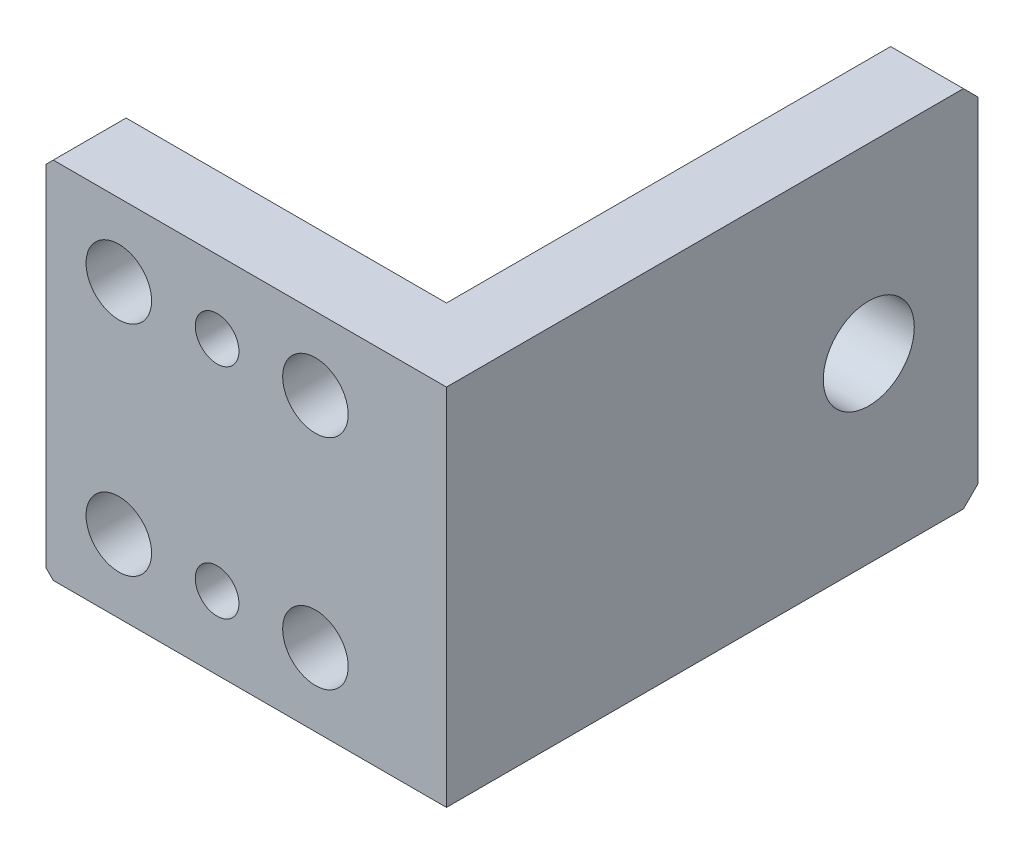
from build123d import *

# Parameters (mm, degrees)
SKETCH1_W                    = 55
SKETCH1_H                    = 50
BOSS_EXTRUDE1_DEPTH          = 10
SKETCH4_W                    = 10
SKETCH4_H                    = 50
BOSS_EXTRUDE2_DEPTH          = 63
M8_CLEARANCE_HOLE1_D         = 9
M8_CLEARANCE_HOLE1_DEPTH     = 121
M8_CLEARANCE_HOLE1_TIP       = 2.703872786
CHAMFER1_SIZE                = 1
M14X1_5_TAPPED_HOLE1_D       = 12.5
CHAMFER2_SIZE                = 2
SIZE_MM_BLIND_DOWEL_HOLE_1_D = 6


with BuildPart() as part:
    # Sketch1 → Boss-Extrude1 (new body)
    with BuildSketch(Plane.XY):
        Rectangle(SKETCH1_W, SKETCH1_H)
    extrude(amount=BOSS_EXTRUDE1_DEPTH)

    # Sketch4 → Boss-Extrude2 (add)
    with BuildSketch(Plane(origin=(0, 0, 0), x_dir=(-1, 0, 0), z_dir=(0, 0, -1))):
        with Locations((-22.5, 0)):
            Rectangle(SKETCH4_W, SKETCH4_H)
    extrude(amount=BOSS_EXTRUDE2_DEPTH)

    # M8 Clearance Hole1
    with Locations(Plane(origin=(0, 0, 0), x_dir=(-1, 0, 0), z_dir=(0, 0, -1))):
        with Locations((17.5, -15), (17.5, 15), (-9.5, -15), (-9.5, 15)):
            Hole(M8_CLEARANCE_HOLE1_D / 2, depth=M8_CLEARANCE_HOLE1_DEPTH)
            with Locations((0, 0, -(M8_CLEARANCE_HOLE1_DEPTH + M8_CLEARANCE_HOLE1_TIP / 2))):  # 118° drill point
                Cone(0, M8_CLEARANCE_HOLE1_D / 2, M8_CLEARANCE_HOLE1_TIP, mode=Mode.SUBTRACT)

    # Chamfer1
    chamfer1_edges = [part.edges().sort_by_distance(p)[0] for p in [
        (-27.5, -25, 5),
        (-27.5, 25, 5),
    ]]
    chamfer(chamfer1_edges, length=CHAMFER1_SIZE)

    # M14x1.5 Tapped Hole1 (through all)
    with Locations(Plane(origin=(27.5, 0, 0), x_dir=(0, 0, -1), z_dir=(1, 0, 0))):
        with Locations((48, 0)):
            Hole(M14X1_5_TAPPED_HOLE1_D / 2)

    # Chamfer2
    chamfer2_edges = [part.edges().sort_by_distance(p)[0] for p in [
        (22.5, 25, -63),
        (22.5, -25, -63),
    ]]
    chamfer(chamfer2_edges, length=CHAMFER2_SIZE)

    # Size mm blind dowel hole 1 (through all)
    with Locations(Plane(origin=(0, 0, 0), x_dir=(-1, 0, 0), z_dir=(0, 0, -1))):
        with Locations((4, -15), (4, 15)):
            Hole(SIZE_MM_BLIND_DOWEL_HOLE_1_D / 2)


solid = part.part
